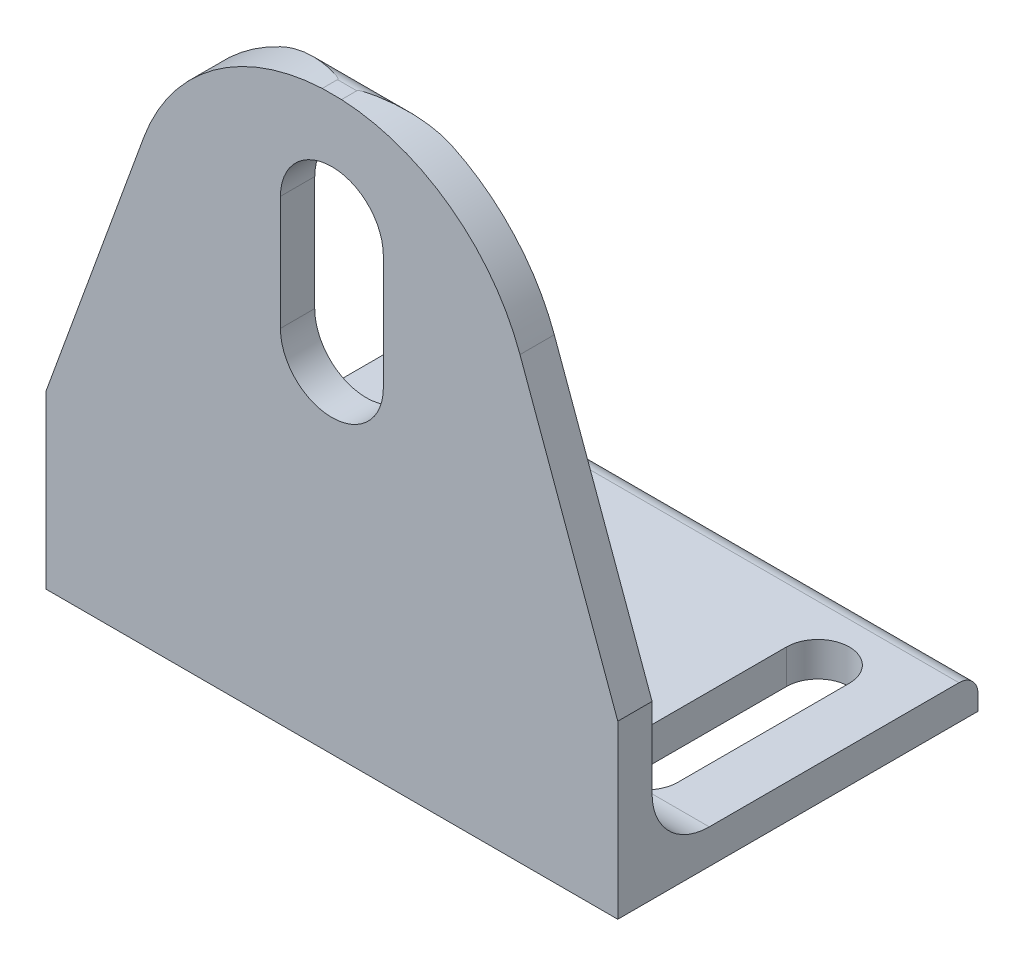
from build123d import *

# Parameters (mm, degrees)
HOT_ROLLED_UNEQUAL_ANGLE_GB_T706_2008_10_DEPTH = 100
SKETCH3_OUTSIDE_W                              = 132.964
SKETCH3_OUTSIDE_H                              = 132.964
CUT_EXTRUDE1_DEPTH                             = 10
CUT_EXTRUDE2_DEPTH                             = 15


with BuildPart() as part:
    # Sketch1 → Hot-rolled unequal angle gb∕t706-2008 100 X 63 X 6(1) (new body)
    with BuildSketch(Plane(origin=(0, 0, 0), x_dir=(0, 0, -1), z_dir=(1, 0, 0))):
        with BuildLine():
            Line((0, 0), (0, 100))
            Line((0, 100), (2.666666667, 100))
            ThreePointArc((2.666666667, 100), (5.023689271, 99.023689271), (6, 96.666666667))
            Line((6, 96.666666667), (6, 16))
            ThreePointArc((6, 16), (8.928932188, 8.928932188), (16, 6))
            Line((16, 6), (59.666666667, 6))
            ThreePointArc((59.666666667, 6), (62.023689271, 5.023689271), (63, 2.666666667))
            Line((63, 2.666666667), (63, 0))
            Line((63, 0), (0, 0))
        make_face()
    extrude(amount=HOT_ROLLED_UNEQUAL_ANGLE_GB_T706_2008_10_DEPTH)

    # Sketch3 outside → Cut-Extrude1 (cut)
    # profile 1 of 2: a face of its own
    with BuildSketch(Plane.XY):
        with Locations((50, 50)):
            Rectangle(SKETCH3_OUTSIDE_W, SKETCH3_OUTSIDE_H)
        with BuildLine():
            Line((0, 30), (17.101007166, 76.984631039))
            ThreePointArc((17.101007166, 76.984631039), (50, 100.040750994), (82.898992834, 76.984631039))
            Line((82.898992834, 76.984631039), (100, 30))
            Line((100, 30), (100, 0))
            Line((100, 0), (0, 0))
            Line((0, 0), (0, 30))
        make_face(mode=Mode.SUBTRACT)
    # profile 2 of 2: a face of its own
    with BuildSketch(Plane.XY):
        with BuildLine():
            Line((59, 80), (59, 60))
            ThreePointArc((59, 60), (50, 51), (41, 60))
            Line((41, 60), (41, 80))
            ThreePointArc((41, 80), (50, 89), (59, 80))
        make_face()
    extrude(amount=-CUT_EXTRUDE1_DEPTH, mode=Mode.SUBTRACT)

    # Sketch4 → Cut-Extrude2 (cut)
    with BuildSketch(Plane.XZ):
        with BuildLine():
            Line((20.5, -20), (20.5, -50))
            ThreePointArc((20.5, -50), (15, -55.5), (9.5, -50))
            Line((9.5, -50), (9.5, -20))
            ThreePointArc((9.5, -20), (15, -14.5), (20.5, -20))
        make_face()
        with BuildLine():
            Line((79.5, -20), (79.5, -50))
            ThreePointArc((79.5, -50), (85, -55.5), (90.5, -50))
            Line((90.5, -50), (90.5, -20))
            ThreePointArc((90.5, -20), (85, -14.5), (79.5, -20))
        make_face()
    extrude(amount=-CUT_EXTRUDE2_DEPTH, mode=Mode.SUBTRACT)


solid = part.part
